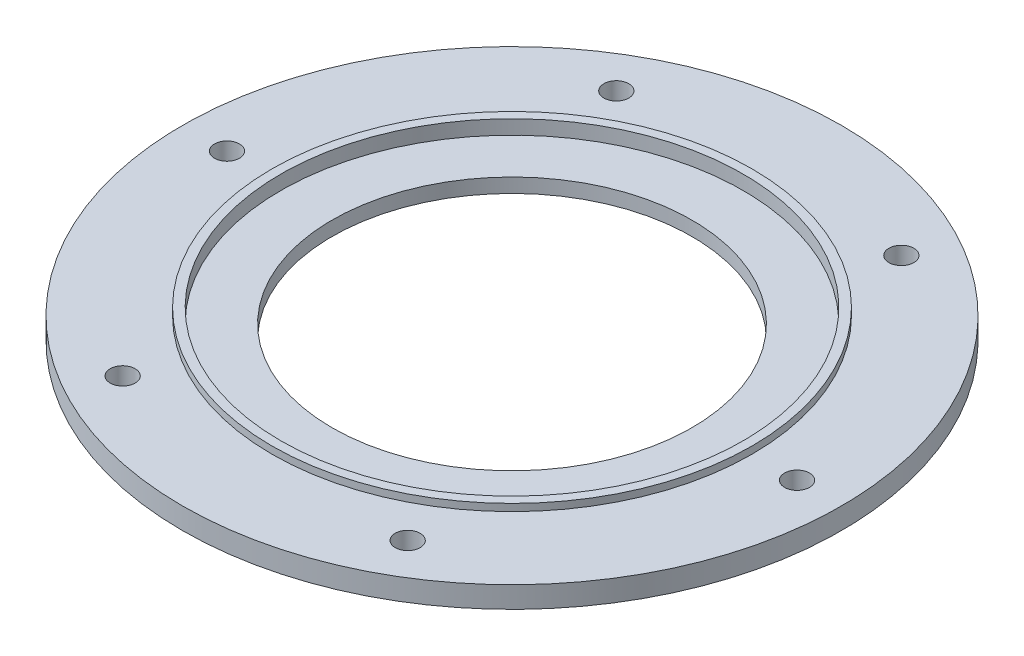
from build123d import *

# Parameters (mm, degrees)
SKETCH1_R           = 185
SKETCH1_R_2         = 101
BOSS_EXTRUDE1_DEPTH = 12
SKETCH2_R           = 129.75
CUT_EXTRUDE1_DEPTH  = 4
BOSS_EXTRUDE2_START = 4
SKETCH3_R           = 134.75
SKETCH3_R_2         = 129.75
BOSS_EXTRUDE2_DEPTH = 4
SKETCH4_R           = 7
CUT_EXTRUDE2_DEPTH  = 262.90456277
CIRPATTERN1_COUNT   = 6


with BuildPart() as part:
    # Sketch1 → Boss-Extrude1 (new body)
    with BuildSketch(Plane(origin=(0, 0, 0), x_dir=(1, 0, 0), z_dir=(0, 1, 0))):
        with Locations(Location((0, 0, 0), (0, 0, 270))):
            Circle(SKETCH1_R)
        with Locations(Location((0, 0, 0), (0, 0, 270))):
            Circle(SKETCH1_R_2, mode=Mode.SUBTRACT)
    extrude(amount=BOSS_EXTRUDE1_DEPTH)

    # Sketch2 → Cut-Extrude1 (cut)
    with BuildSketch(Plane(origin=(0, 12, 0), x_dir=(1, 0, 0), z_dir=(0, 1, 0))):
        with Locations(Location((0, 0, 0), (0, 0, 270))):
            Circle(SKETCH2_R)
    extrude(amount=-CUT_EXTRUDE1_DEPTH, mode=Mode.SUBTRACT)

    # Sketch3 → Boss-Extrude2 (add)
    with BuildSketch(Plane(origin=(0, 12, 0), x_dir=(1, 0, 0), z_dir=(0, 1, 0)).offset(BOSS_EXTRUDE2_START)):
        with Locations(Location((0, 0, 0), (0, 0, 270))):
            Circle(SKETCH3_R)
        with Locations(Location((0, 0, 0), (0, 0, 270))):
            Circle(SKETCH3_R_2, mode=Mode.SUBTRACT)
    extrude(amount=-BOSS_EXTRUDE2_DEPTH)

    # Sketch4 → Cut-Extrude2 (cut, through all)
    with BuildSketch(Plane(origin=(0, 12, 0), x_dir=(1, 0, 0), z_dir=(0, 1, 0))):
        with Locations(Location((160, 0, 0), (0, 0, 270))):
            Circle(SKETCH4_R)
    cut_extrude2 = extrude(amount=-CUT_EXTRUDE2_DEPTH, mode=Mode.SUBTRACT)

    # CirPattern1: Cut-Extrude2 ×6 about axis
    cirpattern1_axis = Axis((0, 0, 0), (0, 1, 0))
    for i in range(1, CIRPATTERN1_COUNT):
        add(cut_extrude2.rotate(cirpattern1_axis, i * 360 / CIRPATTERN1_COUNT), mode=Mode.SUBTRACT)


solid = part.part
